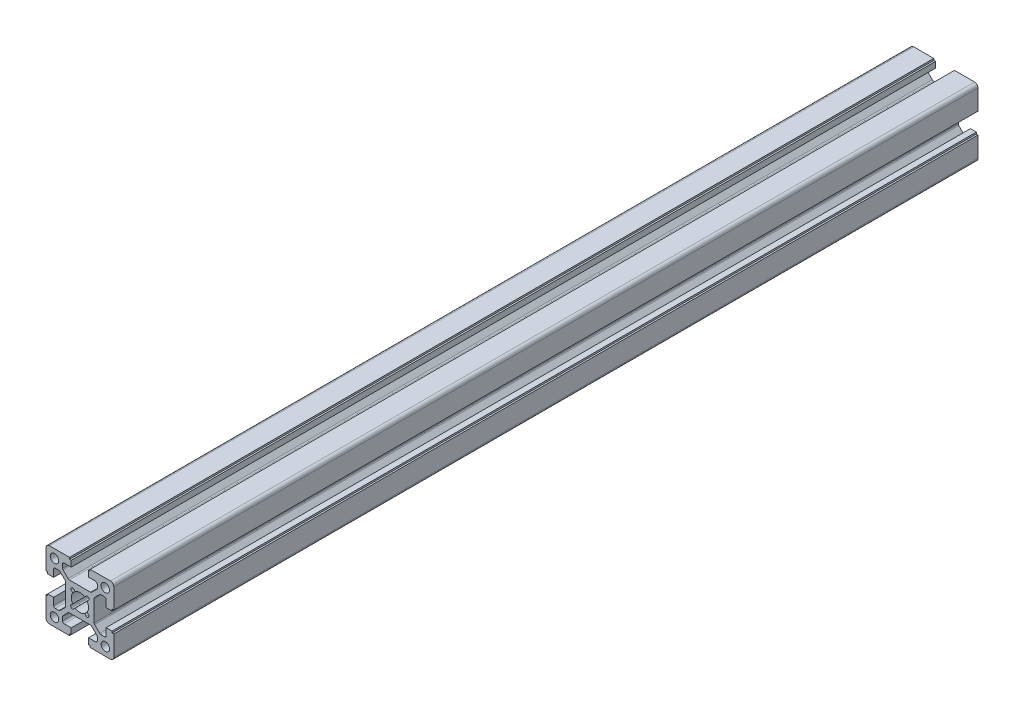
SolidWorks part; units mm, degrees
ref_plane "Front Plane" through (0, 0, 0) normal (0, 0, 1) x (1, 0, 0)
ref_plane "Top Plane" through (0, 0, 0) normal (0, 1, 0) x (1, 0, 0)
ref_plane "Right Plane" through (0, 0, 0) normal (1, 0, 0) x (0, 0, -1)
sketch "Sketch1" plane through (0, 0, 0) normal (0, 0, 1) x (1, 0, 0)
  line L0 (-5.1792, 3.7656) -> (-4.2435, 2.8299)
  line L1 (-4.2435, -2.8281) -> (-5.2772, -3.8618)
  line L2 (-5.2772, -4.9224) -> (-4.924, -5.2756)
  line L3 (-3.8637, -5.276) -> (-2.8295, -4.2431)
  line L4 (2.8295, -4.2431) -> (3.7786, -5.1922)
  line L5 (4.8389, -5.1925) -> (5.193, -4.8389)
  line L6 (5.1933, -3.7779) -> (4.2435, -2.8281)
  line L7 (4.2435, 2.8299) -> (5.1933, 3.7797)
  line L8 (5.1933, 4.8403) -> (4.8393, 5.1943)
  line L9 (3.7783, 5.1939) -> (2.8295, 4.2439)
  line L10 (-2.8295, 4.2439) -> (-3.7652, 5.1796)
  line L11 (-4.8258, 5.1796) -> (-5.1792, 4.8262)
  line L12 (-5.1005, 15.5009) -> (-5.1005, 19.0009)
  line L13 (-9.2505, 15.5009) -> (-5.1005, 15.5009)
  line L14 (-10.2505, 12.4331) -> (-10.2505, 14.5009)
  line L15 (-6.9254, 8.6938) -> (-9.9576, 11.726)
  line L16 (6.2183, 8.4009) -> (-6.2183, 8.4009)
  line L17 (9.9566, 11.725) -> (6.9254, 8.6938)
  line L18 (10.2495, 14.5009) -> (10.2495, 12.4321)
  line L19 (5.0995, 15.5009) -> (9.2495, 15.5009)
  line L20 (5.0995, 19.0009) -> (5.0995, 15.5009)
  line L21 (6.0995, 19.0009) -> (5.0995, 19.0009)
  line L22 (6.0995, 20.0009) -> (6.0995, 19.0009)
  line L23 (17.9995, 20.0009) -> (6.0995, 20.0009)
  line L24 (19.9995, 6.1009) -> (19.9995, 18.0009)
  line L25 (18.9995, 6.1009) -> (19.9995, 6.1009)
  line L26 (18.9995, 5.1009) -> (18.9995, 6.1009)
  line L27 (15.4995, 5.1009) -> (18.9995, 5.1009)
  line L28 (15.4995, 9.2509) -> (15.4995, 5.1009)
  line L29 (12.4317, 10.2509) -> (14.4995, 10.2509)
  line L30 (8.6924, 6.9258) -> (11.7246, 9.958)
  line L31 (8.3995, -6.2169) -> (8.3995, 6.2187)
  line L32 (11.7246, -9.9562) -> (8.6924, -6.924)
  line L33 (14.4995, -10.2491) -> (12.4317, -10.2491)
  line L34 (15.4995, -5.0991) -> (15.4995, -9.2491)
  line L35 (18.9995, -5.0991) -> (15.4995, -5.0991)
  line L36 (18.9995, -6.0991) -> (18.9995, -5.0991)
  line L37 (19.9995, -6.0991) -> (18.9995, -6.0991)
  line L38 (19.9995, -17.9991) -> (19.9995, -6.0991)
  line L39 (6.0995, -19.9991) -> (17.9995, -19.9991)
  line L40 (6.0995, -18.9991) -> (6.0995, -19.9991)
  line L41 (5.0995, -18.9991) -> (6.0995, -18.9991)
  line L42 (5.0995, -15.4991) -> (5.0995, -18.9991)
  line L43 (9.2495, -15.4991) -> (5.0995, -15.4991)
  line L44 (10.2495, -12.4303) -> (10.2495, -14.4991)
  line L45 (6.9254, -8.692) -> (9.9566, -11.7232)
  line L46 (-6.2183, -8.3991) -> (6.2183, -8.3991)
  line L47 (-9.9576, -11.7242) -> (-6.9254, -8.692)
  line L48 (-10.2505, -14.4991) -> (-10.2505, -12.4313)
  line L49 (-5.1005, -15.4991) -> (-9.2505, -15.4991)
  line L50 (-5.1005, -18.9991) -> (-5.1005, -15.4991)
  line L51 (-6.1005, -18.9991) -> (-5.1005, -18.9991)
  line L52 (-6.1005, -19.9991) -> (-6.1005, -18.9991)
  line L53 (-18.0005, -19.9991) -> (-6.1005, -19.9991)
  line L54 (-20.0005, -6.0991) -> (-20.0005, -17.9991)
  line L55 (-19.0005, -6.0991) -> (-20.0005, -6.0991)
  line L56 (-19.0005, -5.0991) -> (-19.0005, -6.0991)
  line L57 (-15.5005, -5.0991) -> (-19.0005, -5.0991)
  line L58 (-15.5005, -9.2491) -> (-15.5005, -5.0991)
  line L59 (-12.4317, -10.2491) -> (-14.5005, -10.2491)
  line L60 (-8.6934, -6.925) -> (-11.7246, -9.9562)
  line L61 (-8.4005, 6.2197) -> (-8.4005, -6.2179)
  line L62 (-11.7246, 9.958) -> (-8.6934, 6.9268)
  line L63 (-14.5005, 10.2509) -> (-12.4317, 10.2509)
  line L64 (-15.5005, 5.1009) -> (-15.5005, 9.2509)
  line L65 (-19.0005, 5.1009) -> (-15.5005, 5.1009)
  line L66 (-19.0005, 6.1009) -> (-19.0005, 5.1009)
  line L67 (-20.0005, 6.1009) -> (-19.0005, 6.1009)
  line L68 (-20.0005, 18.0009) -> (-20.0005, 6.1009)
  line L69 (-6.1005, 20.0009) -> (-18.0005, 20.0009)
  line L70 (-6.1005, 19.0009) -> (-6.1005, 20.0009)
  line L71 (-5.1005, 19.0009) -> (-6.1005, 19.0009)
  arc A0 (-5.1792, 4.8262) -> (-5.1792, 3.7656) centre (-4.6488, 4.2959) ccw
  arc A1 (-4.2435, 2.8299) -> (-4.2435, -2.8281) centre (-0.0001, 0.0009) ccw
  arc A2 (-5.2772, -3.8618) -> (-5.2772, -4.9224) centre (-4.7468, -4.3921) ccw
  arc A3 (-4.924, -5.2756) -> (-3.8637, -5.276) centre (-4.3937, -4.7453) ccw
  arc A4 (-2.8295, -4.2431) -> (2.8295, -4.2431) centre (0, 0) ccw
  arc A5 (3.7786, -5.1922) -> (4.8389, -5.1925) centre (4.3089, -4.6619) ccw
  arc A6 (5.193, -4.8389) -> (5.1933, -3.7779) centre (4.663, -4.3083) ccw
  arc A7 (4.2435, -2.8281) -> (4.2435, 2.8299) centre (0.0001, 0.0009) ccw
  arc A8 (5.1933, 3.7797) -> (5.1933, 4.8403) centre (4.6629, 4.31) ccw
  arc A9 (4.8393, 5.1943) -> (3.7783, 5.1939) centre (4.309, 4.6639) ccw
  arc A10 (2.8295, 4.2439) -> (-2.8295, 4.2439) centre (0, 0.0008) ccw
  arc A11 (-3.7652, 5.1796) -> (-4.8258, 5.1796) centre (-4.2955, 4.6492) ccw
  circle A12 centre (-15.0005, 15.0009) radius 2.5
  circle A13 centre (14.9995, -14.9991) radius 2.5
  arc A14 (-9.2505, 15.5009) -> (-10.2505, 14.5009) centre (-9.2505, 14.5009) ccw
  arc A15 (-10.2505, 12.4331) -> (-9.9576, 11.726) centre (-9.2505, 12.4331) ccw
  arc A16 (-6.9254, 8.6938) -> (-6.2183, 8.4009) centre (-6.2183, 9.4009) ccw
  arc A17 (6.2183, 8.4009) -> (6.9254, 8.6938) centre (6.2183, 9.4009) ccw
  arc A18 (9.9566, 11.725) -> (10.2495, 12.4321) centre (9.2495, 12.4321) ccw
  arc A19 (10.2495, 14.5009) -> (9.2495, 15.5009) centre (9.2495, 14.5009) ccw
  arc A20 (19.9995, 18.0009) -> (17.9995, 20.0009) centre (17.9995, 18.0009) ccw
  arc A21 (15.4995, 9.2509) -> (14.4995, 10.2509) centre (14.4995, 9.2509) ccw
  arc A22 (12.4317, 10.2509) -> (11.7246, 9.958) centre (12.4317, 9.2509) ccw
  arc A23 (8.6924, 6.9258) -> (8.3995, 6.2187) centre (9.3995, 6.2187) ccw
  arc A24 (8.3995, -6.2169) -> (8.6924, -6.924) centre (9.3995, -6.2169) ccw
  arc A25 (11.7246, -9.9562) -> (12.4317, -10.2491) centre (12.4317, -9.2491) ccw
  arc A26 (14.4995, -10.2491) -> (15.4995, -9.2491) centre (14.4995, -9.2491) ccw
  arc A27 (17.9995, -19.9991) -> (19.9995, -17.9991) centre (17.9995, -17.9991) ccw
  arc A28 (9.2495, -15.4991) -> (10.2495, -14.4991) centre (9.2495, -14.4991) ccw
  arc A29 (10.2495, -12.4303) -> (9.9566, -11.7232) centre (9.2495, -12.4303) ccw
  arc A30 (6.9254, -8.692) -> (6.2183, -8.3991) centre (6.2183, -9.3991) ccw
  arc A31 (-6.2183, -8.3991) -> (-6.9254, -8.692) centre (-6.2183, -9.3991) ccw
  arc A32 (-9.9576, -11.7242) -> (-10.2505, -12.4313) centre (-9.2505, -12.4313) ccw
  arc A33 (-10.2505, -14.4991) -> (-9.2505, -15.4991) centre (-9.2505, -14.4991) ccw
  arc A34 (-20.0005, -17.9991) -> (-18.0005, -19.9991) centre (-18.0005, -17.9991) ccw
  arc A35 (-15.5005, -9.2491) -> (-14.5005, -10.2491) centre (-14.5005, -9.2491) ccw
  arc A36 (-12.4317, -10.2491) -> (-11.7246, -9.9562) centre (-12.4317, -9.2491) ccw
  arc A37 (-8.6934, -6.925) -> (-8.4005, -6.2179) centre (-9.4005, -6.2179) ccw
  arc A38 (-8.4005, 6.2197) -> (-8.6934, 6.9268) centre (-9.4005, 6.2197) ccw
  arc A39 (-11.7246, 9.958) -> (-12.4317, 10.2509) centre (-12.4317, 9.2509) ccw
  arc A40 (-14.5005, 10.2509) -> (-15.5005, 9.2509) centre (-14.5005, 9.2509) ccw
  arc A41 (-18.0005, 20.0009) -> (-20.0005, 18.0009) centre (-18.0005, 18.0009) ccw
  circle A42 centre (-15.0005, -14.9991) radius 2.5
  circle A43 centre (14.9995, 15.0009) radius 2.5
extrude "Boss-Extrude1" add sketch "Sketch1" along normal mid plane 510
